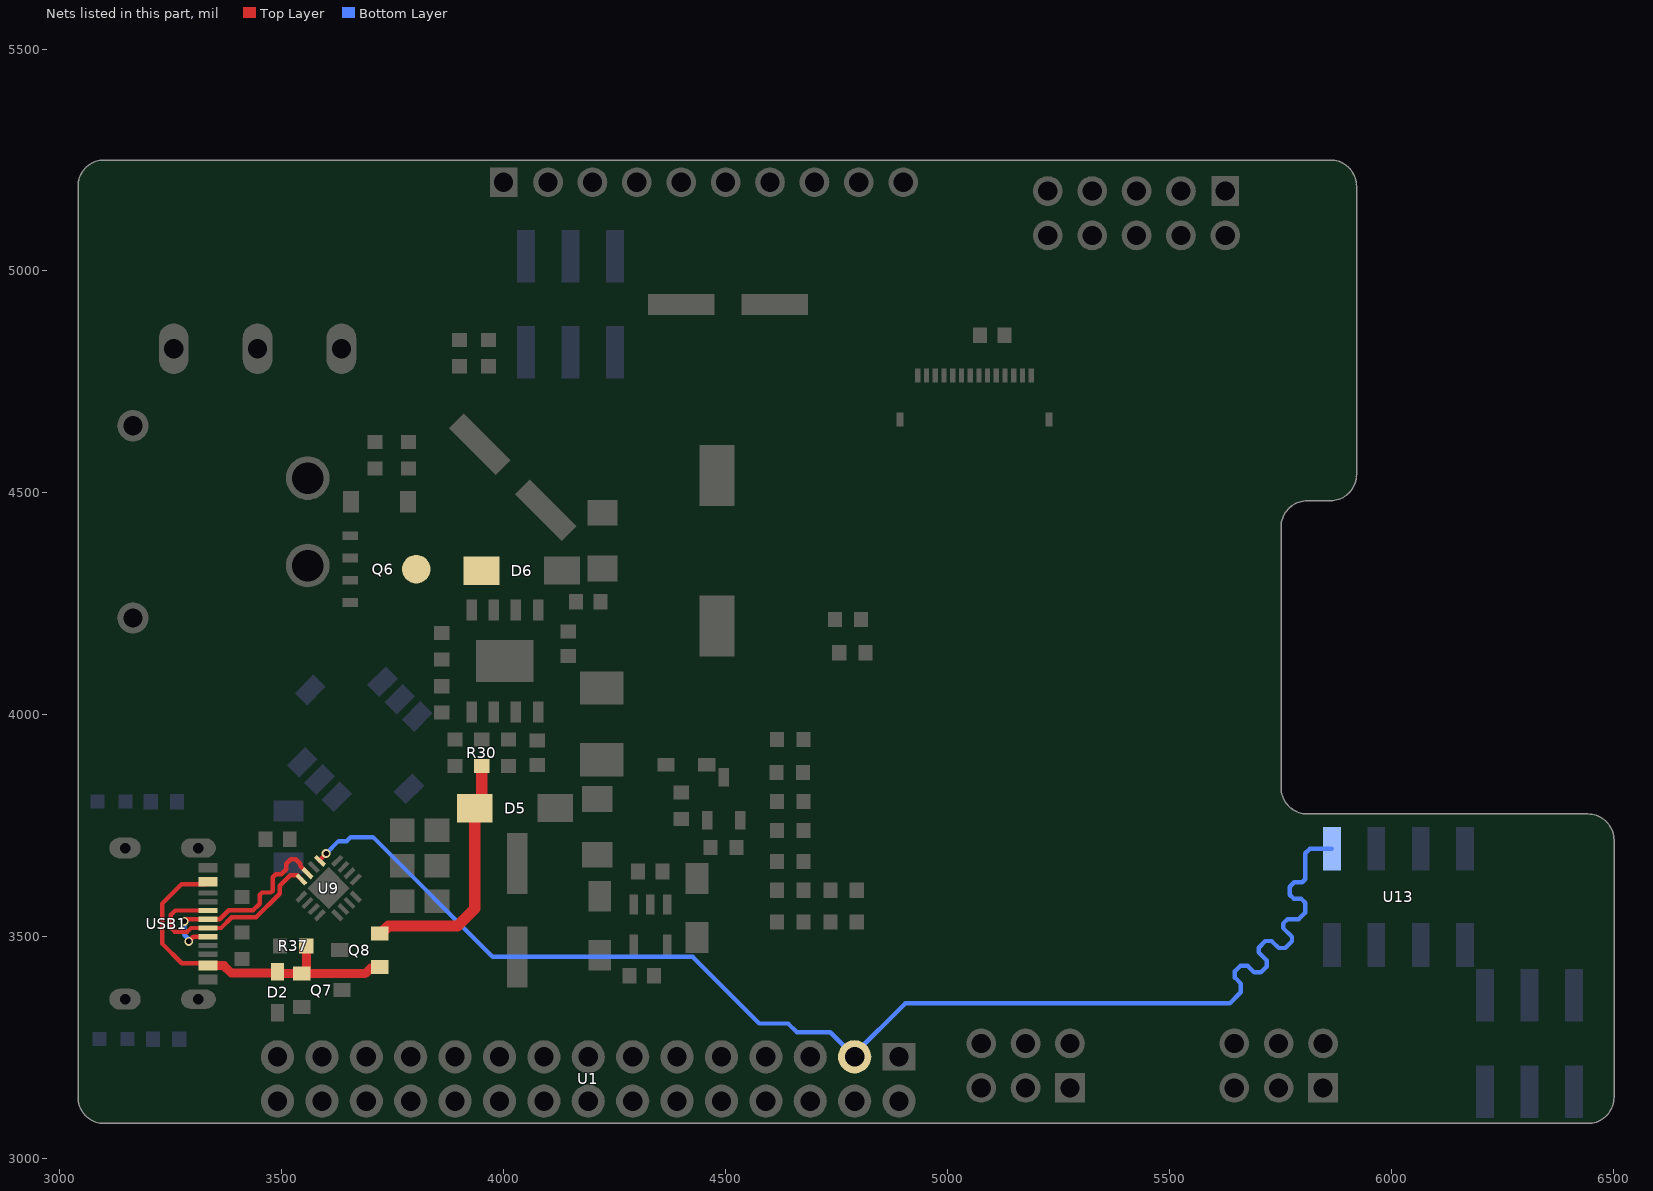
[diagram p0: the nets of this part, all layers, seen from the top]
# Altium PCB MISC51977.pcbdoc (part 3 of 4)
Units mil, origin at the board's own origin, x right, y up, seen from the top; angles counter-clockwise.
Board outline 3460 x 2170.19 mil, 4 copper layers (Top Layer, VCC, GND, Bottom Layer), stack 62.447 mil thick; 74 components, 60 nets, 282 pads, 462 vias.

## Via types
v1: diameter 20, hole 12, Top Layer to Bottom Layer, 455 vias
v2: diameter 24.02, hole 12, Top Layer to Bottom Layer, 7 vias

## Nets (pads, with @x,y where several pads share a name; then routed paths per layer and width w, separated by ;. In a path a pad name is that pad's centre, name@x,y a point inside that pad or via, vN(x,y) a via of type N, cw(c..) or ccw(c..) an arc to the next point about the centre after c; other vN are vias at no path point) (continued)
TX: U1.3 U9.5 U13.1 | length 3007.9
  Top Layer w10: U9.5@3585.51,3671.24 3585.51,3674.03 v1(3599.48,3688)
  Bottom Layer w10: v1(3599.48,3688) 3627.46,3715.98 3645.98,3715.98 3655,3725 3705,3725 3975,3455 4425,3455 4575,3305 4640,3305 4660,3285 4735,3285 U1.3@4790,3230 4790,3236.54 4903.73,3350.28 5635.07,3350.28 5660,3375.21 5660,3395 5646.62,3408.38 5646.62,3422.52 5659.1,3435 5675,3435 5690,3420 5704.79,3420 5717.82,3433.03 5717.82,3447.18 5700,3465 5700,3475.9 5714.98,3490.88 5729.12,3490.88 5745,3475 5759.79,3475 5775.11,3490.32 5775.11,3500.11 5755,3520.21 5755,3530 5765,3540 5790,3540 5804.89,3554.89 5804.89,3577.07 5796.41,3585.54 5779.46,3585.54 5770,3595 5770,3612.93 5780,3622.93 5797.93,3622.93 5804.89,3629.89 5804.89,3688.27 5814.89,3698.27 U13.1@5865,3698.27
UD+: U9.7 USB1.6 USB1.8 | length 485.4
  Top Layer w10: v1(3280,3535) 3284.84,3539.84 USB1.6@3333.51,3539.84 3359.84,3539.84 3380,3560 3435,3560 3450,3575 3450,3595 3455,3600 3475,3600 3479.02,3604.02 3479.02,3634.34 3485.98,3641.3 3498.7,3641.3 3510,3652.61 3510,3665 3520,3675 3531.12,3675 3541.12,3665 3541.12,3659.95 U9.7@3557.67,3643.4 ; v1(3290,3490) 3300.47,3500.47 USB1.8@3333.51,3500.47
  Bottom Layer w10: v1(3280,3535) 3280,3505 3290,3495 v1(3290,3490)
UD-: U9.8 USB1.5 USB1.7 | length 481.1
  Top Layer w10: USB1.5@3333.51,3559.53 3259.53,3559.53 3250,3550 3250,3520 3257.93,3512.07 3287.07,3512.07 3295.16,3520.16 USB1.7@3333.51,3520.16 3362.76,3520.16 3386.62,3544.02 3441.62,3544.02 3495,3597.39 3495,3615 3518.7,3638.7 3534.54,3638.7 U9.8@3543.75,3629.48
VCCBAT: D6.1 Q6.5
VCCBAT_5V: D5.2 Q8.2 R30.2 | length 571
  Top Layer w25: Q8.2@3714.37,3507.4 3722.4,3507.4 3740,3525 3895,3525 3934.3,3564.3 D5.2@3934.3,3789.63 3950,3805.34 R30.2@3950,3885.34
VCCUSB: D2.2 Q7.1 Q8.1 R37.2 USB1.2 USB1.11 | length 797.4
  Top Layer w10: USB1.11@3333.51,3435.51 3319.36,3435.51 3313.89,3440.98 3274.02,3440.98 3230,3485 3230,3575 3274.01,3619.01 3328.03,3619.01 USB1.2@3333.51,3624.49
  Top Layer w20: USB1.11@3333.51,3435.51 3369.35,3435.51 3386.37,3418.48 3487.32,3418.48 D2.2@3490,3421.16 3493.76,3417.4 Q7.1@3555.63,3417.4 ; R37.2@3555,3479.66 3555,3418.03 Q7.1@3555.63,3417.4 ; Q8.1@3714.37,3432.6 3711.77,3430 3700,3430 3687.4,3417.4 Q7.1@3555.63,3417.4
pads on no net: FPC1.1 FPC1.14 H12.3 H12.4 H13.1 H13.2 H14.1 H14.2 SW1.7 SW1.8 U1.1 U2.1 U2.2 U2.3 U2.4 U2.5 U2.6 U2.7 U2.8 U2.9 U2.10 U7.4 U9.10 U9.11 U9.12 U9.13 U9.14 U9.15 U9.16 U13.2 U13.4 U13.6 U13.8 USB1.3 USB1.9
copper on no net: | length 75.7
  Bottom Layer w10: 4665,3905 4700,3905 4728.78,3933.78

## Polygon pours and split planes (outlines as drawn)
+5V on Bottom Layer (solid, remove dead copper, pour order 28): 6120,3755 6120,3555 6210,3555 6210,3755
3V3 on Top Layer (solid, remove dead copper, pour order 16): 5255,4980 5255,4625 5270,4610 5355,4695 5355,4979.76 5354.76,4980
+5V on Top Layer (solid, remove dead copper, pour order 18): 4400,4615 4400,4440 4785,4440 4805,4460 4650,4615
GND on Top Layer (solid, remove dead copper, pour order 26): 3000,5290 3000,3045 6540,3045 6540,5290
VCCBAT on Top Layer (solid, remove dead copper, pour order 22): 3719.29,4420 3945,4420 4005,4360 4005,4273.47 3913.47,4273.47 3905,4265 3905,4228.07 3719.29,4228.07
AGND on GND (solid, remove dead copper): 3380,3719.88 3380,3489.97 3389.97,3480 3455,3480 3487.82,3512.82 3611.6,3512.82 3638.78,3540 3800,3540 3800,3770 3430.12,3770
AGND on GND (solid, remove dead copper): 3716.42,3548.58 3720,3545 3810,3544.73 3810,3775 3805,3780 3720,3780 3716.42,3776.42
GND on Top Layer (solid, remove dead copper, pour order 20): 3775,4145 3901.72,4145 3931.72,4175 4065,4175 4070,4170 4070,4065.14 4015.14,4065.14 3995,4045 3775,4045
AGND on Bottom Layer (solid, remove dead copper, pour order 30): 3447.47,3747.95 3783.2,3747.95 3810,3721.15 3810,3550 3805,3545 3735,3545 3699.66,3509.66 3444.66,3509.66 3444.66,3745.14
GND on GND (solid, remove dead copper): 3005,5275 3005,3030 6550,3030 6550,5275
$2N1742 on Top Layer (solid, remove dead copper, pour order 0): 4045,4550 4170.31,4550 4174.13,4546.18 4174.13,4407.24 4188.66,4392.7 4277.3,4392.7 4280,4390 4280,4285 4275,4280 4195,4280 4190,4275 4190,4220 4185,4215 4105,4215 4100,4220 4100,4263.78 4093.78,4270 4055,4270 4055,4221.87 4035.27,4202.14 3962.86,4202.14 3950,4215 3950,4255 3960,4265 4002,4265 4010.46,4273.47 4010.46,4515.46
$2N1744 on Top Layer (solid, remove dead copper, pour order 2): 4085,4055 4085,4129.7 4115.31,4160 4305,4160 4330,4135 4330,3980 4059.67,3980 4059.67,4029.67
+5V on Top Layer (solid, remove dead copper, pour order 24): 4325,4950 4325,4894.1 4427,4792.1 4493.05,4792.1 4493.05,4949.76 4492.81,4950
$2N1752 on Top Layer (solid, remove dead copper, pour order 4): 4002.12,3841.53 4110.43,3841.53 4117.64,3848.75 4117.64,3962.64 4120,3965 4325,3965 4330,3960 4330,3755 4310,3735 4180,3735 4160,3715 4160,3555 3990,3555 3985,3560 3985,3824.41
$2N1748 on Top Layer (solid, remove dead copper, pour order 6): 3835,4035 3945,4035 3950,4030 3950,3978.3 3941.24,3969.53 3923.99,3969.53 3923.99,3933.99 3911.74,3921.74 3835,3921.74
GND on Bottom Layer (solid, remove dead copper, pour order 32): 3010,5310 3010,3000 6555,3000 6555,5310
+5V on Top Layer (solid, remove dead copper, pour order 8): 4170,3625 4275,3625 4305,3595 4305,3515 4180,3515 4170,3525
+5V on Top Layer (solid, remove dead copper, pour order 10): 3980.01,3282.37 3594.31,3282.37 3594.31,3280.08 3386.61,3280.08 3386.61,3387.69 3581.62,3387.69 3589.31,3380 3589.31,3365.53 3594.31,3360.53 3594.31,3356.93 3695,3356.93 3695,3400 3710,3415 3745,3415 3750,3420 3750,3435 3755,3440 3980.01,3440
3V3 on Top Layer (solid, remove dead copper, pour order 12): 4310,3365.31 4310,3484.89 4361.03,3535.92 4566.38,3535.92 4566.38,3474.6 4485,3474.6 4485,3440.9 4414.88,3365.31
$1N4144 on Top Layer (solid, remove dead copper, pour order 14): 3230,4335 3230,4686.94 3190,4726.94 3190,4950 3370,4950 3370,4770.39 3455,4685.43 3455,4495.43 3530.24,4420.19 3670,4420.19 3670,4235 3330,4235

## Keep-outs
GND:
  region: 4117.64,4086.3 4117.64,3873.7 4322.36,3873.7 4322.36,4086.3
Bottom Layer:
  region: 4117.64,4086.3 4117.64,3873.7 4322.36,3873.7 4322.36,4086.3
  region: 4117.64,4086.3 4117.64,3873.7 4322.36,3873.7 4322.36,4086.3
VCC:
  region: 4117.64,4086.3 4117.64,3873.7 4322.36,3873.7 4322.36,4086.3
Board Outline Layer:
  region: 4555.79,3430 ccw(c4555.79,3395.63) 4521.42,3395.63 ccw(c4555.79,3395.63) 4555.79,3361.26 5574.41,3361.26 ccw(c5574.41,3395.63) 5608.78,3395.63 ccw(c5574.41,3395.63) 5574.41,3430
  region: 4555.79,3430 ccw(c4555.79,3395.63) 4521.42,3395.63 ccw(c4555.79,3395.63) 4555.79,3361.26 5574.41,3361.26 ccw(c5574.41,3395.63) 5608.78,3395.63 ccw(c5574.41,3395.63) 5574.41,3430
  lines w0.1: 4521.42,3395.63 cw(c4555.79,3395.63) 4555.79,3430 5574.41,3430 cw(c5574.41,3395.63) 5608.78,3395.63 cw(c5574.41,3395.63) 5574.41,3361.26 4555.79,3361.26 cw(c4555.79,3395.63) 4521.42,3395.63
  lines w10: 3040.6,3138.86 3040.6,5190.94 cw(c3099.66,5190.94) 3099.66,5250 5861.54,5250 cw(c5861.54,5190.94) 5920.6,5190.94 5920.6,4541.56 cw(c5861.54,4541.56) 5861.54,4482.5 5809.66,4482.5 ccw(c5809.66,4423.44) 5750.6,4423.44 5750.6,3836.09 ccw(c5809.66,3836.09) 5809.66,3777.04 6441.54,3777.04 cw(c6441.54,3717.98) 6500.6,3717.98 6500.6,3138.86 cw(c6441.54,3138.86) 6441.54,3079.81 3099.66,3079.81 cw(c3099.66,3138.86) 3040.6,3138.86

## Other copper
Top Layer:
  drawing of 179 lines, arcs and shapes, not listed
GND:
  region net BUZZER: 4822.61,3169.68 4829.68,3162.61 4827.66,3160.41 4826.14,3158.34 4825.04,3156.37 4824.33,3154.48 4823.95,3152.64 4823.86,3150.82 4824,3148.99 4824.32,3147.14 4825.3,3143.22 4826.41,3138.86 4826.87,3136.44 4827.22,3133.83 4827.39,3131 4827.34,3127.92 4787.92,3167.34 4791,3167.39 4793.83,3167.22 4796.44,3166.87 4798.86,3166.41 4803.22,3165.3 4807.14,3164.32 4808.99,3164 4810.82,3163.86 4812.64,3163.95 4814.48,3164.33 4816.37,3165.04 4818.34,3166.14 4820.41,3167.66
  region net KEY_RIGHT: 4550.32,3262.61 4557.39,3269.68 4559.59,3267.66 4561.66,3266.14 4563.63,3265.04 4565.52,3264.33 4567.36,3263.95 4569.18,3263.86 4571.01,3264 4572.86,3264.32 4576.78,3265.3 4581.14,3266.41 4583.56,3266.87 4586.17,3267.22 4589,3267.39 4592.08,3267.34 4552.66,3227.92 4552.61,3231 4552.78,3233.83 4553.13,3236.44 4553.59,3238.86 4554.7,3243.22 4555.68,3247.14 4556,3248.99 4556.14,3250.82 4556.05,3252.64 4555.67,3254.48 4554.96,3256.37 4553.86,3258.34 4552.34,3260.41
  region net KEY_LEFT: 4485,3281.12 4495,3281.12 4495.13,3278.13 4495.51,3275.59 4496.13,3273.42 4496.97,3271.58 4498,3270.02 4499.22,3268.66 4500.61,3267.47 4502.15,3266.39 4505.61,3264.31 4509.48,3262.01 4511.52,3260.63 4513.61,3259.03 4515.74,3257.15 4517.88,3254.93 4462.12,3254.93 4464.26,3257.15 4466.39,3259.03 4468.48,3260.63 4470.52,3262.01 4474.39,3264.31 4477.85,3266.39 4479.39,3267.47 4480.78,3268.66 4482,3270.02 4483.03,3271.58 4483.87,3273.42 4484.49,3275.59 4484.87,3278.13
  region net KEY_MID: 4322.61,3169.68 4329.68,3162.61 4327.66,3160.41 4326.14,3158.34 4325.04,3156.37 4324.33,3154.48 4323.95,3152.64 4323.86,3150.82 4324,3148.99 4324.32,3147.14 4325.3,3143.22 4326.41,3138.86 4326.87,3136.44 4327.22,3133.83 4327.39,3131 4327.34,3127.92 4287.92,3167.34 4291,3167.39 4293.83,3167.22 4296.44,3166.87 4298.86,3166.41 4303.22,3165.3 4307.14,3164.32 4308.99,3164 4310.82,3163.86 4312.64,3163.95 4314.48,3164.33 4316.37,3165.04 4318.34,3166.14 4320.41,3167.66
  region net I2C_SCL: 4150.32,3262.61 4157.39,3269.68 4159.59,3267.66 4161.66,3266.14 4163.63,3265.04 4165.52,3264.33 4167.36,3263.95 4169.18,3263.86 4171.01,3264 4172.86,3264.32 4176.78,3265.3 4181.14,3266.41 4183.56,3266.87 4186.17,3267.22 4189,3267.39 4192.08,3267.34 4152.66,3227.92 4152.61,3231 4152.78,3233.83 4153.13,3236.44 4153.59,3238.86 4154.7,3243.22 4155.68,3247.14 4156,3248.99 4156.14,3250.82 4156.05,3252.64 4155.67,3254.48 4154.96,3256.37 4153.87,3258.34 4152.34,3260.41
  region net I2C_SDA: 4122.61,3269.68 4129.68,3262.61 4127.66,3260.41 4126.14,3258.34 4125.04,3256.37 4124.33,3254.48 4123.95,3252.64 4123.86,3250.82 4124,3248.99 4124.32,3247.14 4125.3,3243.22 4126.41,3238.86 4126.87,3236.44 4127.22,3233.83 4127.39,3231 4127.34,3227.92 4087.92,3267.34 4091,3267.39 4093.83,3267.22 4096.44,3266.87 4098.86,3266.41 4103.22,3265.3 4107.14,3264.32 4108.99,3264 4110.82,3263.86 4112.64,3263.95 4114.48,3264.33 4116.37,3265.04 4118.34,3266.14 4120.41,3267.66
  region net KEY_UP: 3691.16,3285.37 3701.16,3276.18 3701.34,3274.4 3701.83,3272.64 3702.61,3270.91 3703.64,3269.19 3704.88,3267.5 3706.28,3265.83 3709.47,3262.53 3716.26,3256.15 3719.26,3253.05 3720.53,3251.52 3721.61,3250 3666.61,3259.19 3671.19,3262.49 3675.63,3265.22 3679.78,3267.65 3683.49,3270.07 3685.14,3271.36 3686.63,3272.77 3687.94,3274.31 3689.05,3276.03 3689.95,3277.95 3690.61,3280.13 3691.02,3282.59
  region net BUZZER: 4655.7,3780 4657.19,3770 4655.36,3769.8 4653.41,3769.25 4651.6,3768.38 4650.19,3767.25 4648.7,3782.08 4650.21,3781.24 4652.05,3780.58 4653.97,3780.15
  region net KEY_RIGHT: 4760,3701.33 4750,3701.33 4749.82,3703.1 4749.31,3705.04 4748.53,3706.87 4747.55,3708.33 4762.45,3708.33 4761.47,3706.87 4760.69,3705.04 4760.18,3703.1
  region net KEY_MID: 4725,3735.35 4715,3735.35 4714.82,3737.12 4714.31,3739.05 4713.53,3740.89 4712.55,3742.35 4727.45,3742.35 4726.47,3740.89 4725.69,3739.05 4725.18,3737.12
  region net KEY_UP: 3709.81,3982.74 3706.47,3993.54 3708.94,3996.1 3709.99,3997.48 3710.86,3999.05 3716.99,3985.46 3716.03,3985.66 3715.06,3985.65 3714.1,3985.46 3713.15,3985.12 3711.37,3984.08
  region net $1N4273: 6361.33,3360 6361.33,3370 6363.1,3370.18 6365.04,3370.69 6366.87,3371.47 6368.33,3372.45 6368.33,3357.55 6366.87,3358.53 6365.04,3359.31 6363.1,3359.82
  region net 3V3: 4594.36,4154.07 4601.43,4161.14 4602.81,4160.02 4604.54,4159.02 4606.39,4158.27 4608.12,4157.93 4597.58,4147.39 4597.23,4149.12 4596.49,4150.96 4595.48,4152.69
  region net I2C_SCL: 4730.98,3976.33 4720.98,3976.33 4720.8,3978.1 4720.29,3980.04 4719.51,3981.87 4718.53,3983.33 4733.44,3983.33 4732.46,3981.87 4731.68,3980.04 4731.17,3978.1
  region net I2C_SDA: 4705,3976.33 4695,3976.33 4694.82,3978.1 4694.31,3980.04 4693.53,3981.87 4692.55,3983.33 4707.45,3983.33 4706.47,3981.87 4705.69,3980.04 4705.18,3978.1
  region net 3V3: 3299.54,3858.21 3309.54,3858.21 3309.73,3856.44 3310.24,3854.5 3311.01,3852.67 3312,3851.21 3297.09,3851.21 3298.07,3852.67 3298.85,3854.5 3299.36,3856.44